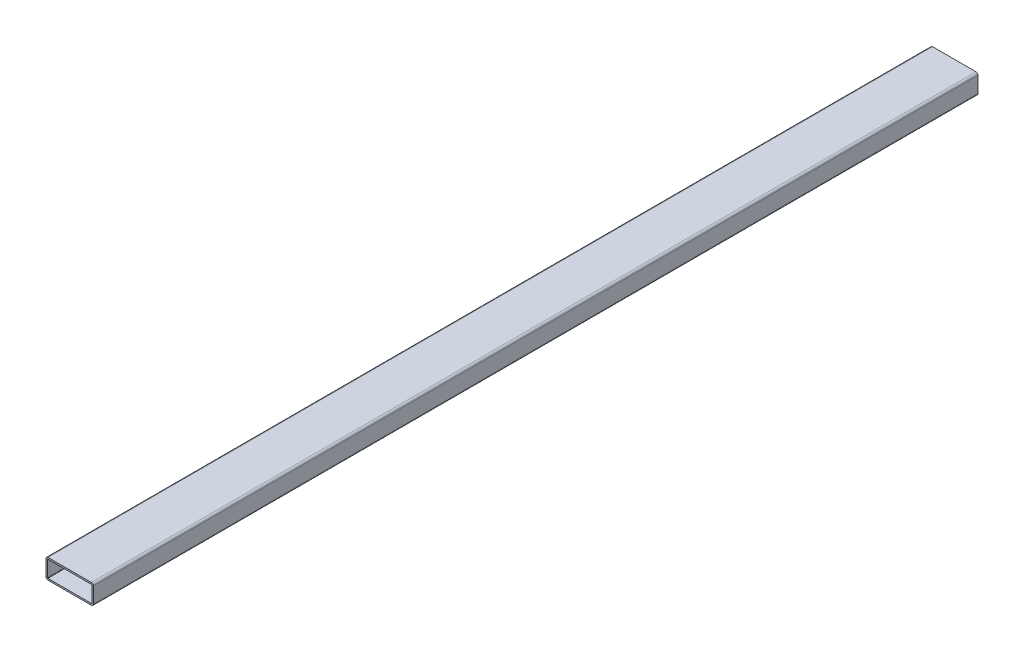
SolidWorks part; units mm, degrees
material "1023 Carbon Steel Plate (SS)"
ref_plane "Front Plane" through (0, 0, 0) normal (0, 0, 1) x (1, 0, 0)
ref_plane "Top Plane" through (0, 0, 0) normal (0, 1, 0) x (1, 0, 0)
ref_plane "Right Plane" through (0, 0, 0) normal (1, 0, 0) x (0, 0, -1)
sketch "Sketch1" plane through (0, 0, 0) normal (0, 0, 1) x (1, 0, 0)
  line L1 (55, 25) -> (-55, 25)
  line L2 (60, 20) -> (60, -20)
  line L3 (55, -25) -> (-55, -25)
  line L4 (-60, 20) -> (-60, -20)
  line L5 (60, 25) -> (-60, -25) construction
  line L6 (60, -25) -> (-60, 25) construction
  arc A0 (-55, -25) -> (-60, -20) centre (-55, -20) cw
  arc A1 (60, -20) -> (55, -25) centre (55, -20) cw
  arc A2 (55, 25) -> (60, 20) centre (55, 20) cw
  arc A3 (-55, 25) -> (-60, 20) centre (-55, 20) ccw
  point P0 (0, 0)
  dimension "D3" = 5
  dimension "D1" = 120
  dimension "D2" = 50
extrude "Boss-Extrude1" add sketch "Sketch1" along normal blind 2240 contours L4 A0 L3 A1 L2 A2 L1 A3
shell "Shell1" thickness 4
